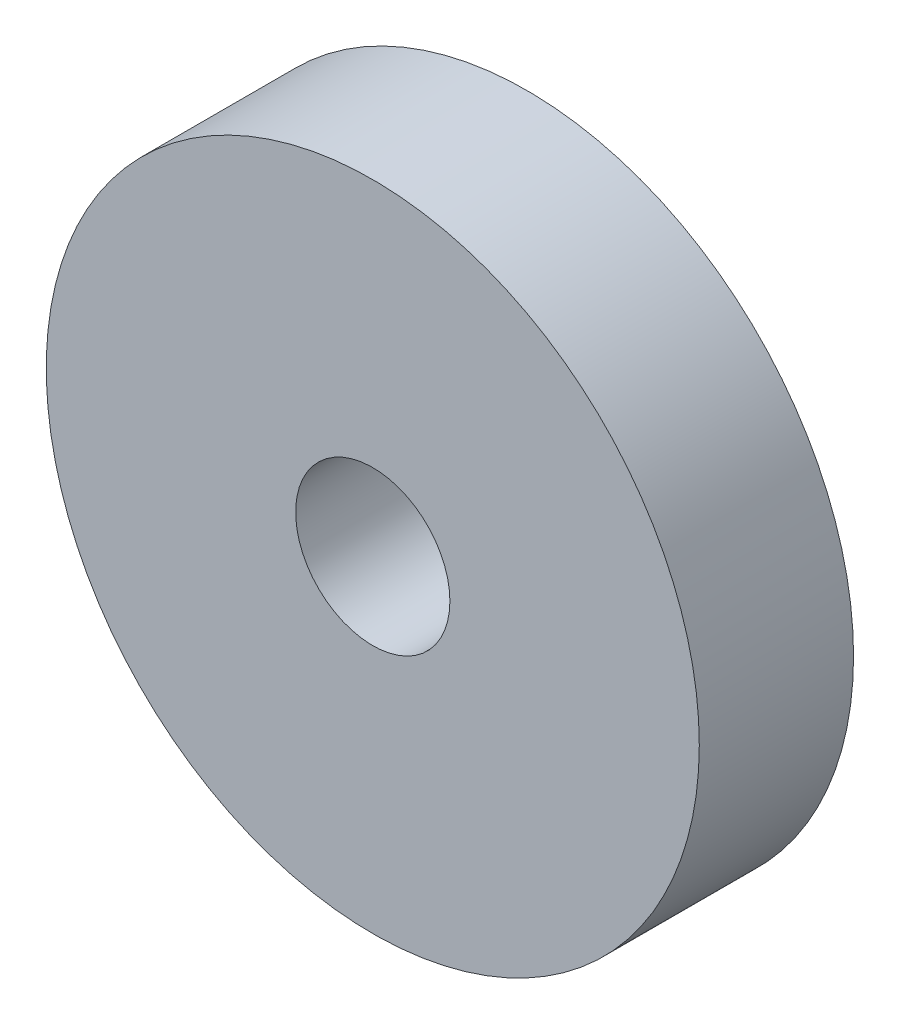
SolidWorks part; units mm, degrees
ref_plane "Front Plane" through (0, 0, 0) normal (0, 0, 1) x (1, 0, 0)
ref_plane "Top Plane" through (0, 0, 0) normal (0, 1, 0) x (1, 0, 0)
ref_plane "Right Plane" through (0, 0, 0) normal (1, 0, 0) x (0, 0, -1)
other "Configuration Table"
sketch "Sketch1" plane through (0, 0, 0) normal (0, 0, 1) x (1, 0, 0)
  circle A0 centre (0, 0) radius 12.7
  circle A1 centre (0, 0) radius 3
  dimension "D1" = 25.4
  dimension "D2" = 6
extrude "Boss-Extrude1" add sketch "Sketch1" along normal blind 6
